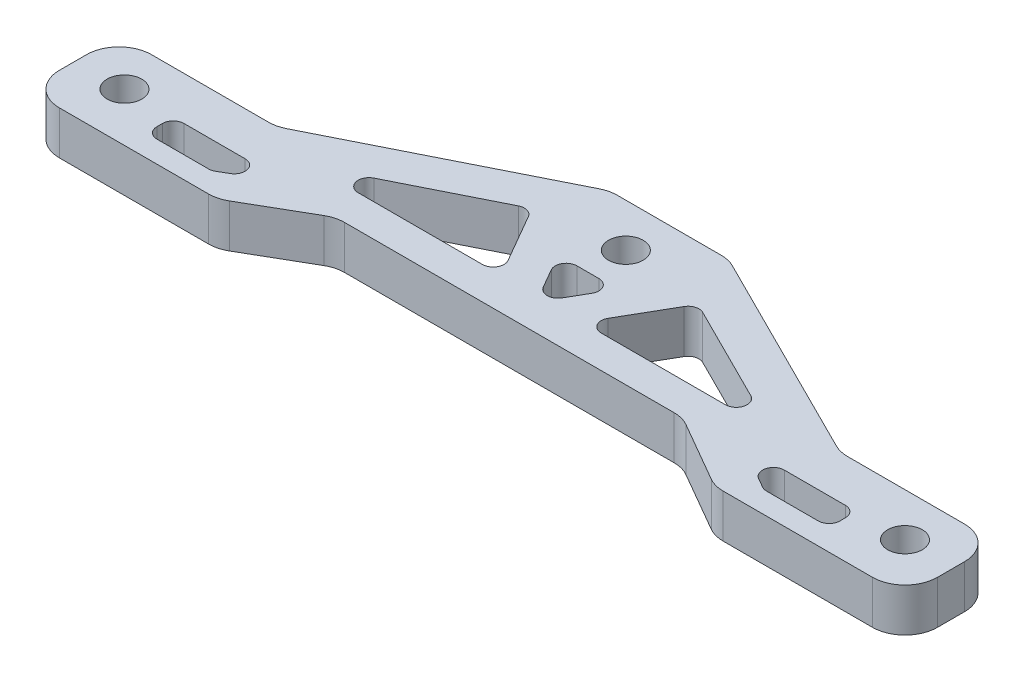
from build123d import *

# Parameters (mm, degrees)
SKETCH_1_R          = 1.6
EXTRUDE_1_DEPTH     = 4
CUT_EXTRUDE_1_DEPTH = 44.119746057
FILLET_R1_R         = 1
FILLET_R3_R         = 3


with BuildPart() as part:
    # 草图1 → 凸台-拉伸1 (new body)
    with BuildSketch(Plane(origin=(0, 0, 0), x_dir=(1, 0, 0), z_dir=(0, 1, 0))):
        Polygon((-40.5, -4.5), (-22.92820323, -4.5), (-16, -0.5), (16, -0.5), (22.92820323, -4.5), (40.5, -4.5), (40.5, 4), (26, 4), (5.5, 14.25), (-5.5, 14.25), (-26, 4), (-40.5, 4), align=None)
        with Locations(Location((-36, 0, 0), (0, 0, 270))):
            Circle(SKETCH_1_R, mode=Mode.SUBTRACT)
        with Locations(Location((36, 0, 0), (0, 0, 270))):
            Circle(SKETCH_1_R, mode=Mode.SUBTRACT)
        with Locations(Location((0, 10.25, 0), (0, 0, 270))):
            Circle(SKETCH_1_R, mode=Mode.SUBTRACT)
    extrude(amount=EXTRUDE_1_DEPTH)

    # 草图2 → 切除-拉伸1 (cut, through all)
    with BuildSketch(Plane(origin=(0, 4, 0), x_dir=(1, 0, 0), z_dir=(0, 1, 0))):
        Polygon((-7.655238394, 9.259261842), (-21.173762079, 2.5), (-3.75277675, 2.5), align=None)
        Polygon((-2.742413779, 6.75), (0, 2), (2.742413779, 6.75), align=None)
        Polygon((21.173762079, 2.5), (3.75277675, 2.5), (7.655238394, 9.259261842), align=None)
        Polygon((-31.5, 0), (-21.133974596, 0), (-25.464101615, -2.5), (-31.5, -2.5), align=None)
        Polygon((25.464101615, -2.5), (31.5, -2.5), (31.5, 0), (21.133974596, 0), align=None)
    extrude(amount=-CUT_EXTRUDE_1_DEPTH, mode=Mode.SUBTRACT)

    # R1 镂空圆角
    fillet_r1_edges = [part.edges().sort_by_distance(p)[0] for p in [
        (-25.464101615, 2, 2.5),
        (-31.5, 2, 2.5),
        (-31.5, 2, 0),
        (-21.133974596, 2, 0),
        (25.464101615, 2, 2.5),
        (21.133974596, 2, 0),
        (31.5, 2, 0),
        (31.5, 2, 2.5),
        (7.655238394, 2, -9.259261842),
        (21.173762079, 2, -2.5),
        (3.75277675, 2, -2.5),
        (-2.742413779, 2, -6.75),
        (2.742413779, 2, -6.75),
        (0, 2, -2),
        (-7.655238394, 2, -9.259261842),
        (-3.75277675, 2, -2.5),
        (-21.173762079, 2, -2.5),
    ]]
    fillet(fillet_r1_edges, radius=FILLET_R1_R)

    # R3 外缘圆角
    fillet_r3_edges = [part.edges().sort_by_distance(p)[0] for p in [
        (40.5, 2, -4),
        (40.5, 2, 4.5),
        (22.92820323, 2, 4.5),
        (16, 2, 0.5),
        (-16, 2, 0.5),
        (-22.92820323, 2, 4.5),
        (-40.5, 2, 4.5),
        (-40.5, 2, -4),
        (-26, 2, -4),
        (-5.5, 2, -14.25),
        (5.5, 2, -14.25),
        (26, 2, -4),
    ]]
    fillet(fillet_r3_edges, radius=FILLET_R3_R)


solid = part.part
